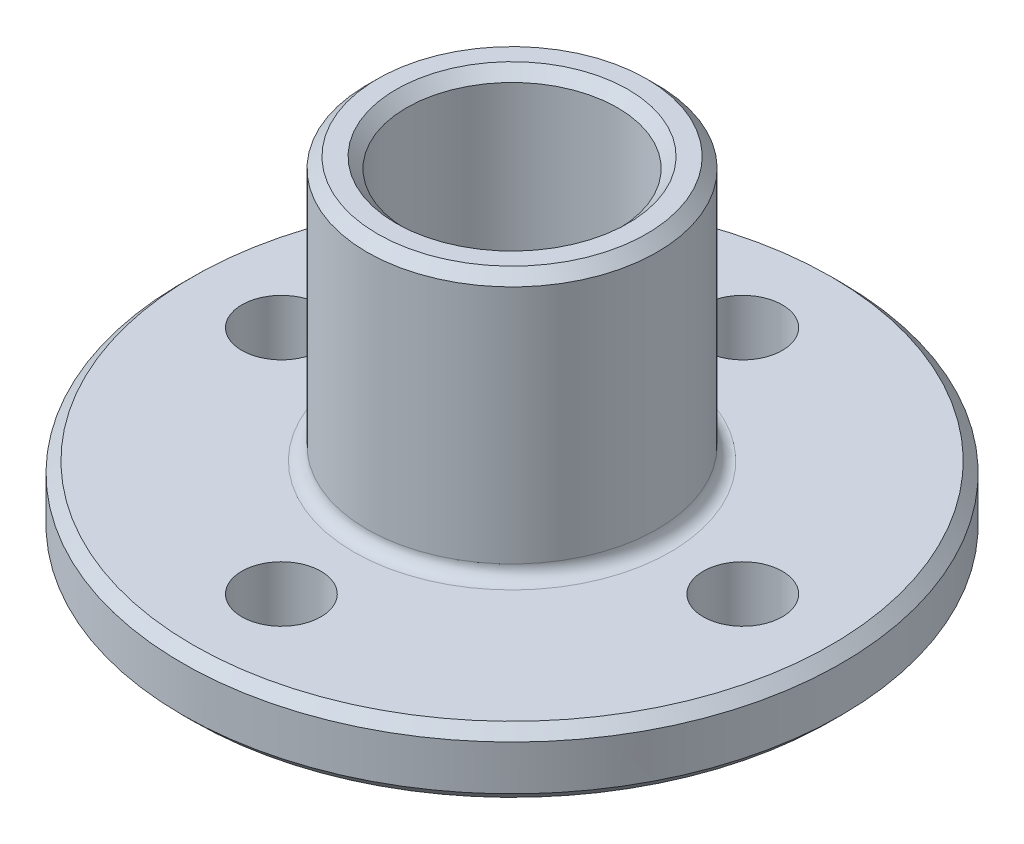
from build123d import *

# Parameters (mm, degrees)
SKETCH1_R           = 25
BOSS_EXTRUDE2_DEPTH = 5
SKETCH3_R           = 3
CUT_EXTRUDE2_DEPTH  = 5
SKETCH4_R           = 11
SKETCH4_R_2         = 8
BOSS_EXTRUDE3_DEPTH = 20
CHAMFER1_SIZE       = 0.8
FILLET1_R           = 1


with BuildPart() as part:
    # Sketch1 → Boss-Extrude2 (new body)
    with BuildSketch(Plane(origin=(0, 0, 0), x_dir=(1, 0, 0), z_dir=(0, 1, 0))):
        with Locations(Location((0, 0, 0), (0, 0, 270))):
            Circle(SKETCH1_R)
    extrude(amount=BOSS_EXTRUDE2_DEPTH)

    # Sketch3 → Cut-Extrude2 (cut)
    with BuildSketch(Plane(origin=(0, 0, 0), x_dir=(1, 0, 0), z_dir=(0, 1, 0))):
        with Locations(Location((-17.5, 0, 0), (0, 0, 270))):
            Circle(SKETCH3_R)
        with Locations(Location((0, 17.5, 0), (0, 0, 270))):
            Circle(SKETCH3_R)
        with Locations(Location((17.5, 0, 0), (0, 0, 270))):
            Circle(SKETCH3_R)
        with Locations(Location((0, -17.5, 0), (0, 0, 270))):
            Circle(SKETCH3_R)
    extrude(amount=CUT_EXTRUDE2_DEPTH, mode=Mode.SUBTRACT)

    # Sketch4 → Boss-Extrude3 (add)
    with BuildSketch(Plane(origin=(0, 5, 0), x_dir=(1, 0, 0), z_dir=(0, 1, 0))):
        with Locations(Location((0, 0, 0), (0, 0, 270))):
            Circle(SKETCH4_R)
        with Locations(Location((0, 0, 0), (0, 0, 270))):
            Circle(SKETCH4_R_2, mode=Mode.SUBTRACT)
    extrude(amount=BOSS_EXTRUDE3_DEPTH)

    # Chamfer1
    chamfer1_edges = [part.edges().sort_by_distance(p)[0] for p in [
        (0, 0, -25),
        (0, 25, -11),
        (0, 25, -8),
        (0, 5, -25),
    ]]
    chamfer(chamfer1_edges, length=CHAMFER1_SIZE)

    # Fillet1
    fillet1_edges = [part.edges().sort_by_distance(p)[0] for p in [
        (0, 5, -11),
    ]]
    fillet(fillet1_edges, radius=FILLET1_R)


solid = part.part
